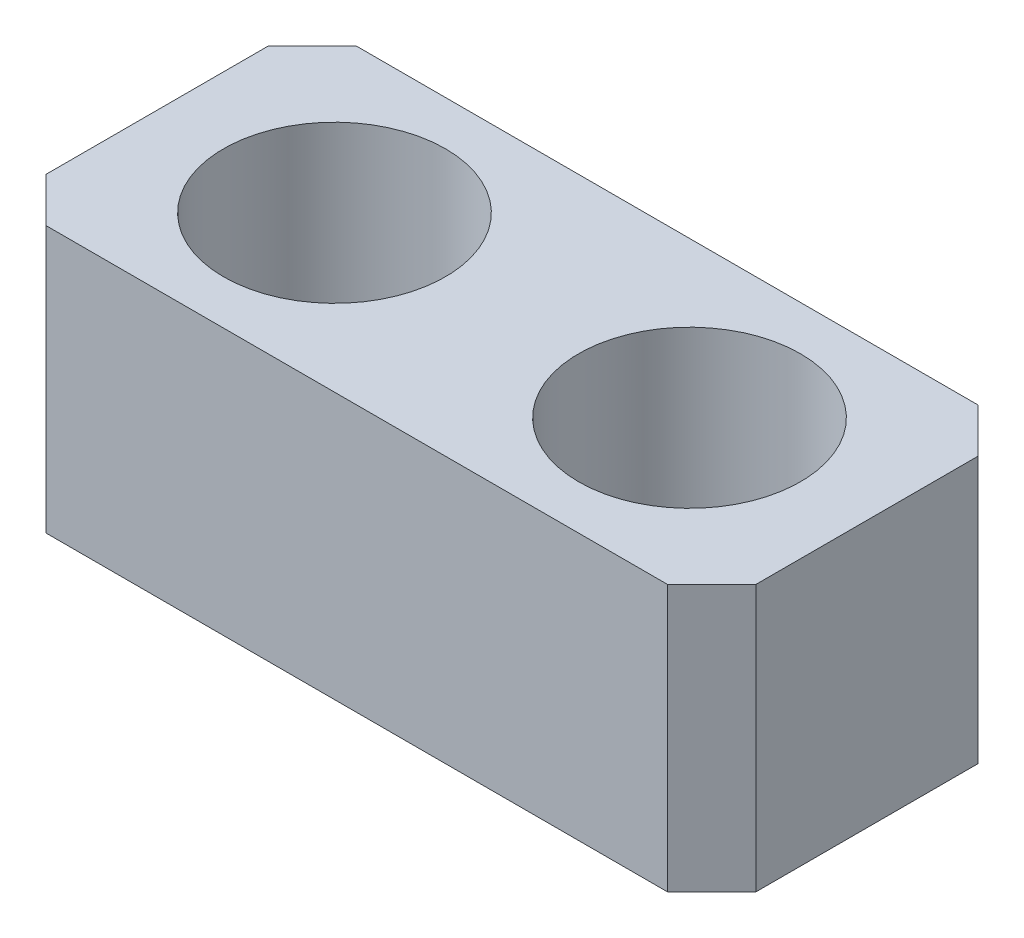
SolidWorks part; units mm, degrees
ref_plane "Front Plane" through (0, 0, 0) normal (0, 0, 1) x (1, 0, 0)
ref_plane "Top Plane" through (0, 0, 0) normal (0, 1, 0) x (1, 0, 0)
ref_plane "Right Plane" through (0, 0, 0) normal (1, 0, 0) x (0, 0, -1)
sketch "Sketch1" plane through (0, 0, 0) normal (0, 1, 0) x (1, 0, 0)
  line L1 (-4, 1.75) -> (4, 1.75)
  line L2 (-4, 1.75) -> (-4, -1.75)
  line L3 (-4, -1.75) -> (4, -1.75)
  line L4 (4, 1.75) -> (4, -1.75)
  line L5 (-4, 1.75) -> (4, -1.75) construction
  line L6 (-4, -1.75) -> (4, 1.75) construction
  point P0 (0, 0)
  dimension "D1" = 8
  dimension "D2" = 3.5
extrude "Boss-Extrude1" add sketch "Sketch1" along normal mid plane 3
sketch "Sketch2" plane through (0, 1.5, 0) normal (0, 1, 0) x (1, 0, 0)
  line L0 (-4, 1.75) -> (-4, -1.75) construction
  circle A0 centre (-2, 0) radius 1.25
  dimension "D1" = 2.5
  dimension "D2" = 2
extrude "Cut-Extrude1" cut sketch "Sketch2" against normal blind 2
chamfer "Chamfer1" distance 0.5 angle 45 4 edges at (4, 0, 1.75) (4, 0, -1.75) (-4, 0, 1.75) (-4, 0, -1.75)
hole_wizard "Ø1.0 (1) Diameter Hole1" positions "Sketch4" profile "Sketch3" hole size "Ø1.0" standard "Gb" end condition through all
sketch "Sketch4" plane through (0, -1.5, 0) normal (0, -1, 0) x (-1, 0, 0)
  point P0 (2, 0)
sketch "Sketch3" plane through (-2, -1.5, 0) normal (1, 0, 0) x (0, 0, -1)
  line L0 (0, 0) -> (0, 3)
  line L1 (0, 3) -> (0.5, 3)
  line L2 (0.5, 3) -> (0.5, 0)
  line L5 (0.5, 0) -> (0, 0)
  line L11 (0, -6.35) -> (0, 107.95) construction
  dimension "通孔孔直径" = 1
  dimension "通孔孔深度" = 3
hole_wizard "Ø2.5 (2.5) Diameter Hole1" positions "Sketch6" profile "Sketch5" hole size "Ø2.5" standard "Gb" end condition through all
sketch "Sketch6" plane through (0, -1.5, 0) normal (0, -1, 0) x (-1, 0, 0)
  line L0 (-4, -1.25) -> (-4, 1.25) construction
  point P0 (-2, 0)
  dimension "D1" = 2
sketch "Sketch5" plane through (2, -1.5, 0) normal (1, 0, 0) x (0, 0, -1)
  line L0 (0, 0) -> (0, 3)
  line L1 (0, 3) -> (1.25, 3)
  line L2 (1.25, 3) -> (1.25, 0)
  line L5 (1.25, 0) -> (0, 0)
  line L11 (0, -6.35) -> (0, 107.95) construction
  dimension "通孔孔直径" = 2.5
  dimension "通孔孔深度" = 3
